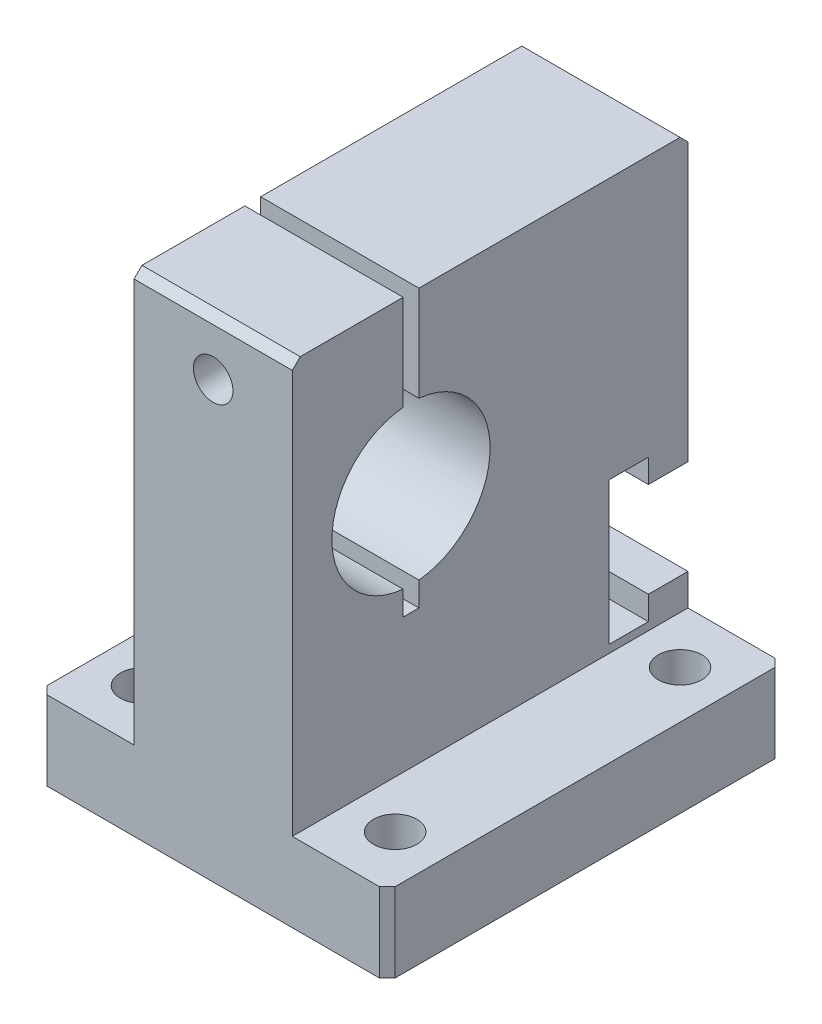
SolidWorks part; units mm, degrees
ref_plane "Front Plane" through (0, 0, 0) normal (0, 0, 1) x (1, 0, 0)
ref_plane "Top Plane" through (0, 0, 0) normal (0, 1, 0) x (1, 0, 0)
ref_plane "Right Plane" through (0, 0, 0) normal (1, 0, 0) x (0, 0, -1)
sketch "Sketch1" plane through (0, 0, 0) normal (0, 0, 1) x (1, 0, 0)
  line L0 (32, 10) -> (44, 10)
  line L1 (0, 0) -> (44, 0)
  line L2 (0, 0) -> (0, 10)
  line L3 (0, 10) -> (12, 10)
  line L4 (44, 0) -> (44, 10)
  line L6 (12, 10) -> (12, 62)
  line L7 (12, 62) -> (32, 62)
  line L8 (32, 10) -> (32, 62)
  dimension "D1" = 10
  dimension "D2" = 44
  dimension "D3" = 20
  dimension "D4" = 62
extrude "Boss-Extrude1" add sketch "Sketch1" along normal blind 50
sketch "Sketch2" plane through (0, 0, 0) normal (0, -1, 0) x (1, 0, 0)
  line L0 (0, 50) -> (0, 0) construction
  line L1 (0, 50) -> (44, 50) construction
  circle A0 centre (6, 43) radius 2.75
  circle A1 centre (6, 7) radius 2.75
  circle A2 centre (38, 43) radius 2.75
  circle A3 centre (38, 7) radius 2.75
  dimension "D1" = 5.5
  dimension "D2" = 36
  dimension "D3" = 32
  dimension "D4" = 6
  dimension "D5" = 7
extrude "Cut-Extrude1" cut sketch "Sketch2" against normal up to next
sketch "Sketch3" plane through (12, 0, 0) normal (-1, 0, 0) x (0, 0, 1)
  line L0 (50, 62) -> (0, 62) construction
  line L1 (0, 62) -> (0, 10) construction
  line L2 (34, 49.9499) -> (34, 62)
  line L3 (34, 62) -> (36, 62)
  line L4 (36, 49.9499) -> (36, 62)
  line L5 (5, 26) -> (5, 29)
  line L6 (0, 14) -> (5, 14)
  line L7 (0, 14) -> (0, 26)
  line L8 (0, 26) -> (5, 26)
  line L9 (50, 0) -> (0, 0) construction
  line L10 (5, 11) -> (10, 11)
  line L11 (5, 11) -> (5, 14)
  line L12 (5, 29) -> (10, 29)
  line L13 (10, 11) -> (10, 29)
  line L14 (35, 40) -> (35, 63.5159) construction
  line L16 (34, 30.0501) -> (34, 27)
  line L17 (34, 27) -> (36, 27)
  line L18 (36, 30.0501) -> (36, 27)
  arc A0 (34, 49.9499) -> (34, 30.0501) centre (35, 40) ccw
  arc A1 (36, 30.0501) -> (36, 49.9499) centre (35, 40) ccw
  dimension "D2" = 10
  dimension "D4" = 22
  dimension "D5" = 35
  dimension "D6" = 18
  dimension "D7" = 12
  dimension "D8" = 5
  dimension "D9" = 5
  dimension "D10" = 14
  dimension "D11" = 35
  dimension "D12" = 2
extrude "Cut-Extrude2" cut sketch "Sketch3" against normal up to next
hole_wizard "Hole size per socket head cap screw type 1" positions "Sketch5" profile "Sketch4" counterbore size "M6" standard "GB"
sketch "Sketch5" plane through (0, 0, 0) normal (0, 0, -1) x (-1, 0, 0)
  line L0 (-12, 62) -> (-12, 26) construction
  line L1 (-32, 62) -> (-12, 62) construction
  point P0 (-22, 55)
  dimension "D1" = 10
  dimension "D2" = 7
sketch "Sketch4" plane through (22, 55, 0) normal (1, 0, 0) x (0, 1, 0)
  line L0 (0, 0) -> (0, 34)
  line L1 (0, 34) -> (3.3, 34)
  line L3 (3.3, 34) -> (3.3, 6.8)
  line L4 (3.3, 6.8) -> (5.5, 6.8)
  line L5 (5.5, 6.8) -> (5.5, 0)
  line L7 (5.5, 0) -> (0, 0)
  line L11 (0, -6.35) -> (0, 107.95) construction
  dimension "通孔孔直径" = 6.6
  dimension "通孔孔深度" = 34
  dimension "柱形沉头孔直径" = 11
  dimension "柱形沉头孔深度" = 6.8
hole_wizard "M6 Tapped Hole1" positions "Sketch7" profile "Sketch8" tap size "M6" standard "GB" end condition through all
sketch "Sketch7" plane through (0, 0, 0) normal (0, 0, -1) x (-1, 0, 0)
  point P0 (-22, 55)
sketch "Sketch8" plane through (22, 55, 0) normal (1, 0, 0) x (0, 1, 0)
  line L0 (0, 0) -> (0, 50)
  line L1 (0, 50) -> (2.5, 50)
  line L2 (2.5, 50) -> (2.5, 0)
  line L5 (2.5, 0) -> (0, 0)
  line L11 (0, -6.35) -> (0, 107.95) construction
  dimension "通孔螺纹孔钻头直径" = 5
  dimension "通孔螺纹孔钻头深度" = 50
cosmetic thread "Cosmetic Thread1" parameters "D2"=6
chamfer "Chamfer1" distance 1 angle 45 6 edges at (22, 62, 50) (22, 62, 0) (0, 5, 0) (0, 5, 50) (44, 5, 50) (44, 5, 0)
